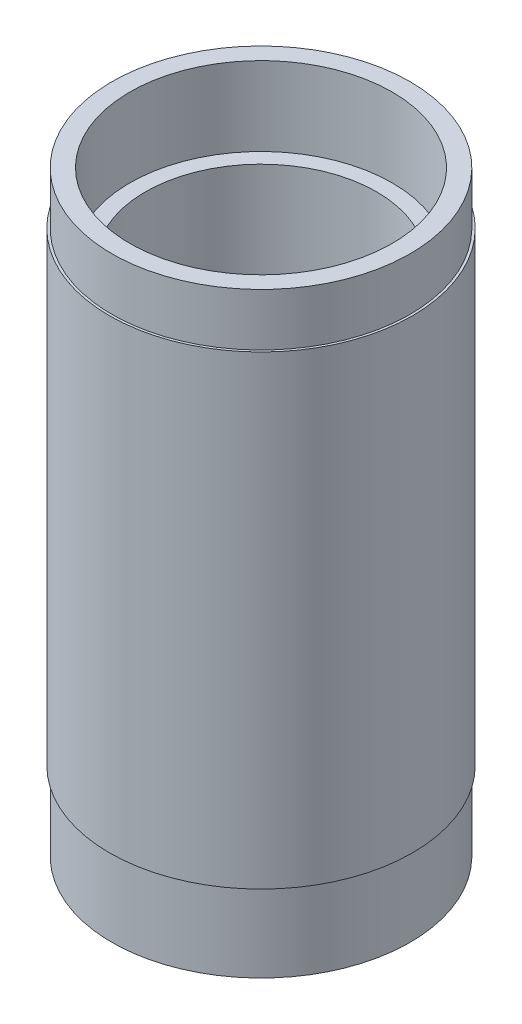
from build123d import *


with BuildPart() as part:
    # Sketch1 → Revolve1 (revolve)
    with BuildSketch(Plane.XY, mode=Mode.PRIVATE) as revolve1_sk:
        Polygon((55, 0), (55, 33), (48.5, 33), (48.5, 217), (55, 217), (55, 250), (62.5, 250), (62.5, 228), (63.5, 228), (63.5, 33), (62.5, 33), (62.5, 0), align=None)
    revolve(revolve1_sk.sketch.rotate(Axis((0, 0, 0), (0, 1, 0)), 90), axis=Axis((0, 0, 0), (0, 1, 0)))


solid = part.part
